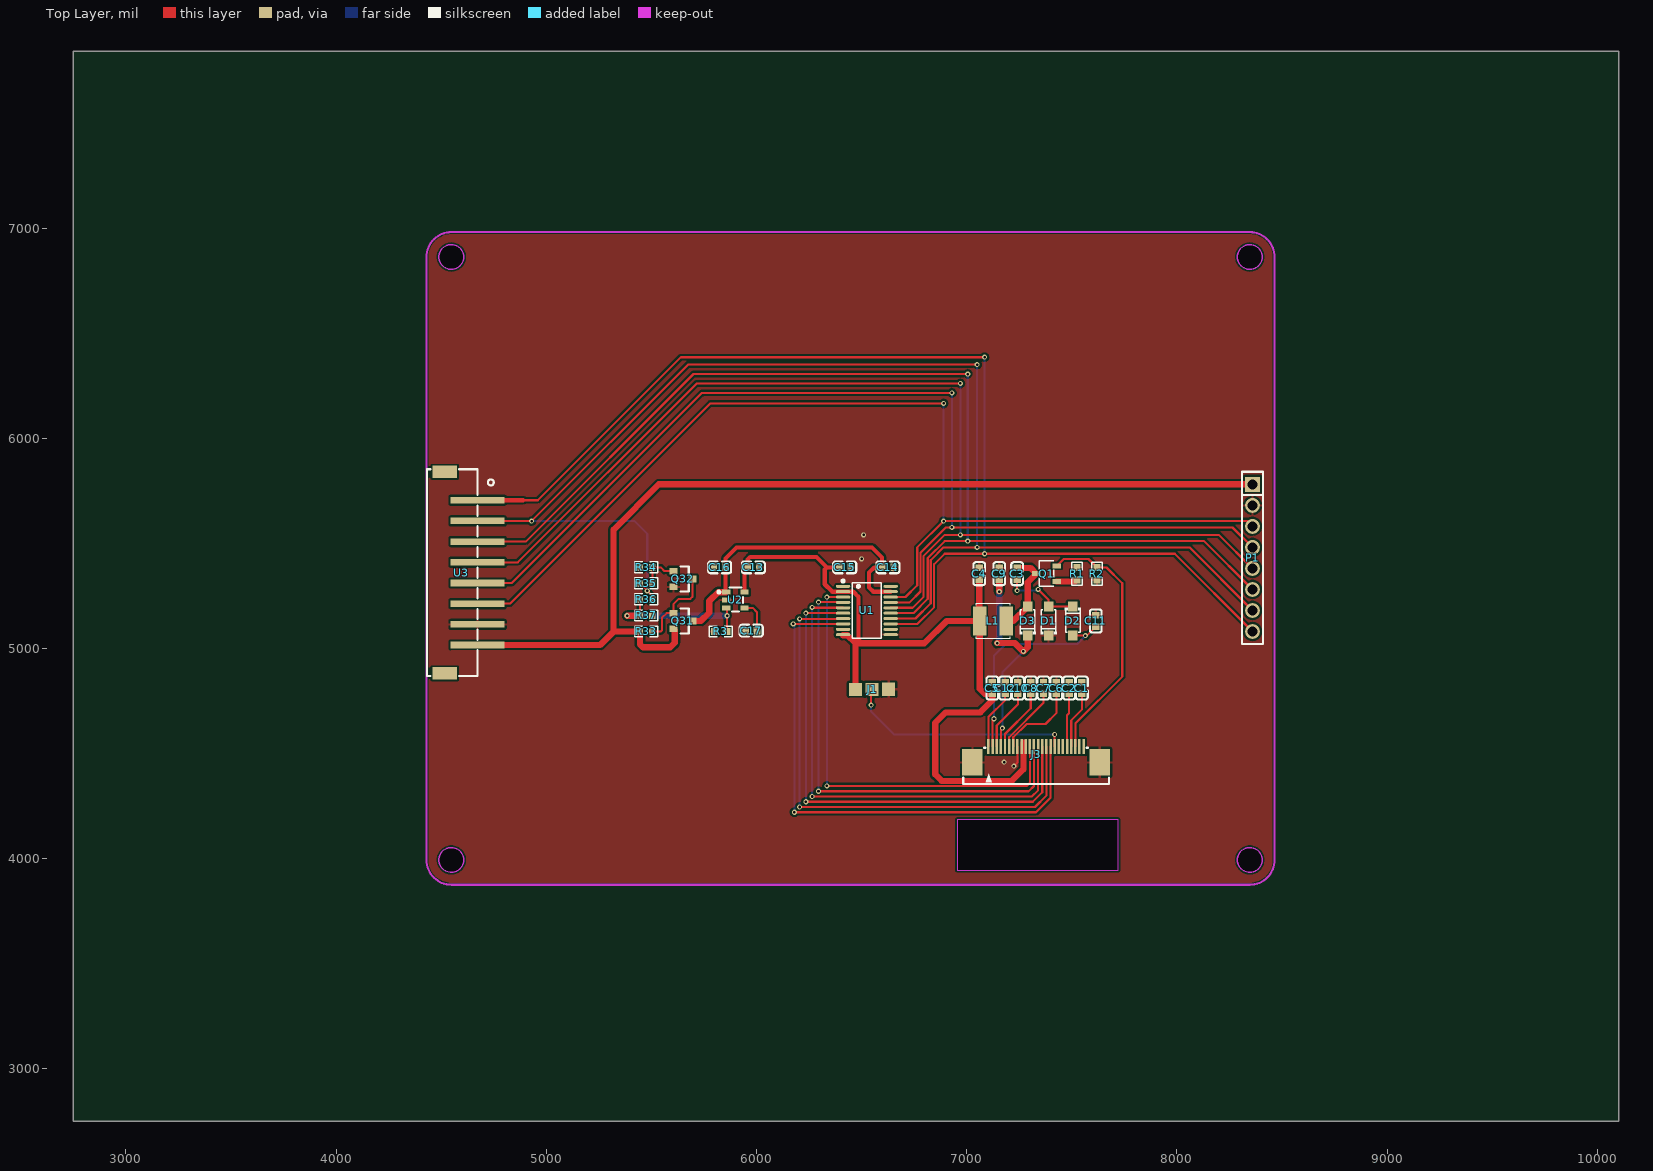
[diagram p0: Top Layer view]
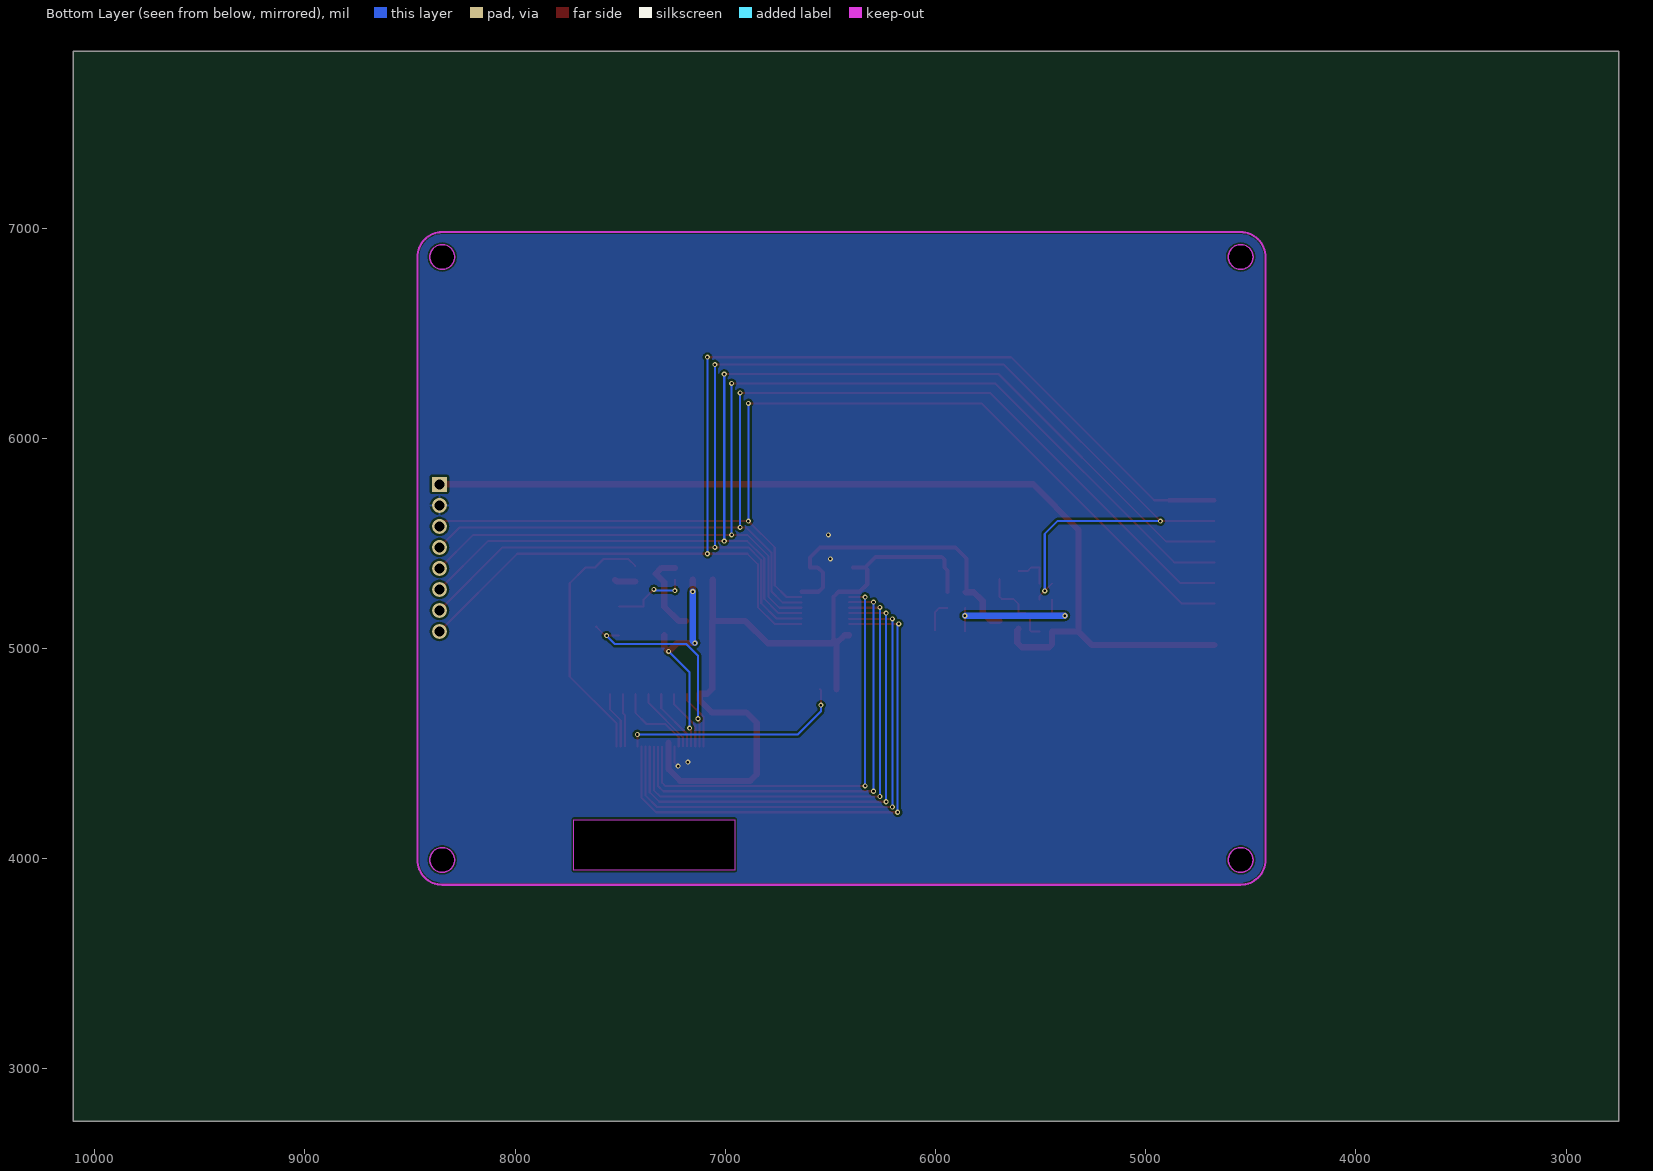
[diagram p1: Bottom Layer view, seen from below]
# Altium PCB MISC61435.pcbdoc
Units mil, origin at the board's own origin, x right, y up, seen from the top; angles counter-clockwise.
Board outline 7351.71 x 5090.35 mil, 2 copper layers (Top Layer, Bottom Layer), stack 62.206 mil thick; 38 components, 35 nets, 139 pads, 42 vias.

## Layer stack, top to bottom
Top Solder Mask Layer: solder mask 0.394, Dk 3.3
Top Layer: signal copper 1.379
Dielectric1: surface 59.449, FR4, Dk 4.5
Bottom Layer: signal copper 1.378
Bottom Solder Mask Layer: solder mask 0.394, Dk 3.3

## Board outline
10101.71,2750 2750,2750 2750,7840.35 10101.71,7840.35
cut-out: 4607.17,3993.46 cw(c4548.11,3993.46) 4489.06,3993.46 cw(c4548.11,3993.46)
cut-out: 8405.94,3993.46 cw(c8346.89,3993.46) 8287.83,3993.46 cw(c8346.89,3993.46)
cut-out: 8405.94,6862.24 cw(c8346.89,6862.24) 8287.83,6862.24 cw(c8346.89,6862.24)
cut-out: 4607.17,6862.24 cw(c4548.11,6862.24) 4489.06,6862.24 cw(c4548.11,6862.24)
cut-out: 6955,4185.35 6955,3945.35 7720,3945.35 7720,4185.35

## Design rules (kind name [scope] priority, off if disabled: settings)
BoardOutlineClearance copperThickness2oz_1 [All] p2 off: genericclearance=7.99 ignorepadtopadclearanceinfootprint=FALSE except(0: Arc-SplitContinuation Track-SplitContinuation SMDPad-SplitContinuation THPad-SplitContinuation Via-SplitContinuation Fill-SplitContinuation Region-SplitContinuation Poly-SplitContinuation Text-SplitContinuation Hole-SplitContinuation; 5.98: Arc-CutoutEdge SMDPad-CutoutEdge THPad-CutoutEdge Via-CutoutEdge Fill-CutoutEdge Region-CutoutEdge Text-CutoutEdge; 6.93: Hole-OutlineEdge Hole-CutoutEdge; 10: Poly-OutlineEdge Poly-CutoutEdge; 11.81: Arc-OutlineEdge Track-OutlineEdge SMDPad-OutlineEdge THPad-OutlineEdge Via-OutlineEdge Fill-OutlineEdge Region-OutlineEdge Text-OutlineEdge Track-CutoutEdge)
BoardOutlineClearance copperThickness1oz_1 [All] p4: genericclearance=4.02 ignorepadtopadclearanceinfootprint=FALSE except(0: Arc-SplitContinuation Track-SplitContinuation SMDPad-SplitContinuation THPad-SplitContinuation Via-SplitContinuation Fill-SplitContinuation Region-SplitContinuation Poly-SplitContinuation Text-SplitContinuation Hole-SplitContinuation; 6: SMDPad-CutoutEdge THPad-CutoutEdge Via-CutoutEdge Fill-CutoutEdge Region-CutoutEdge Text-CutoutEdge; 6.93: Hole-OutlineEdge Hole-CutoutEdge; 10: Poly-OutlineEdge Poly-CutoutEdge; 11.8: Arc-OutlineEdge Track-OutlineEdge SMDPad-OutlineEdge THPad-OutlineEdge Via-OutlineEdge Fill-OutlineEdge Region-OutlineEdge Text-OutlineEdge; 11.81: Arc-CutoutEdge Track-CutoutEdge)
Clearance copperThickness2oz [All] p1 off: gap=7.99 ignorepadtopadclearanceinfootprint=FALSE except(5.98: SMDPad-Track SMDPad-SMDPad THPad-Track SMDPad-THPad THPad-THPad Track-Via SMDPad-Via THPad-Via Via-Via Fill-Track Region-Track Fill-SMDPad Region-SMDPad Fill-THPad Region-THPad Fill-Via Region-Via Fill-Fill Fill-Region Region-Region Arc-Track Arc-SMDPad Arc-THPad Arc-Via Fill-Arc Region-Arc Arc-Arc Text-Track SMDPad-Text Text-THPad Text-Via Fill-Text Region-Text Arc-Text Text-Text; 6.93: Hole-Track Hole-SMDPad Hole-THPad Hole-Via Fill-Hole Region-Hole Hole-Arc Hole-Text; 10: Poly-Track Poly-SMDPad Poly-THPad Poly-Via Poly-Fill Poly-Region Poly-Poly Poly-Arc Poly-Text Poly-Hole)
Clearance copperThickness1oz [All] p3: gap=4.02 ignorepadtopadclearanceinfootprint=FALSE except(5.98: SMDPad-Track SMDPad-SMDPad THPad-Track SMDPad-THPad THPad-THPad Track-Via SMDPad-Via THPad-Via Via-Via Fill-Track Region-Track Fill-SMDPad Region-SMDPad Fill-THPad Region-THPad Fill-Via Region-Via Fill-Fill Fill-Region Region-Region; 6: Arc-Track Arc-SMDPad Arc-THPad Arc-Via Fill-Arc Region-Arc Arc-Arc Text-Track SMDPad-Text Text-THPad Text-Via Fill-Text Region-Text Arc-Text Text-Text; 6.93: Hole-Track Hole-SMDPad Hole-THPad Hole-Via Fill-Hole Region-Hole Hole-Arc Hole-Text; 10: Poly-Track Poly-SMDPad Poly-THPad Poly-Via Poly-Fill Poly-Region Poly-Poly Poly-Arc Poly-Text Poly-Hole)
DiffPairsRouting differentialPair [All] p1: maxlimit=6 minlimit=6 mostfreqgap=6 toplayer_minwidth=5 toplayer_prefwidth=10 toplayer_maxwidth=100 toplayer_mingap=6 toplayer_prefgap=6 toplayer_maxgap=6 bottomlayer_minwidth=5 bottomlayer_prefwidth=10 bottomlayer_maxwidth=100 bottomlayer_mingap=6 bottomlayer_prefgap=6 bottomlayer_maxgap=6 maxuncoupledlength=10
HoleToHoleClearance otherClearance [All] p1: gap=11.81 allowstackedmicrovias=TRUE
Length netLength [All] p1: minlimit=0 maxlimit=0
MatchedLengths netLengthTolerance [All] p1: tolerance=1000
PasteMaskExpansion pasteMaskExpansion [All] p1: expansion=0
PlaneConnect innerPlane [All] p1: planeconnectstyle=Relief reliefexpansion=20 reliefentries=4 reliefconductorwidth=10 reliefairgap=10
PolygonConnect copperRegion [(InNet('GND'))] p1: connectstyle=Relief reliefconductorwidth=10 reliefentries=4 polygonreliefangle="90 Angle" airgapwidth=10 via.connectstyle=Relief via.reliefconductorwidth=10 via.reliefentries=4 via.polygonreliefangle="90 Angle" via.airgapwidth=10
RoutingVias viaSize [All] p1: holewidth=12.01 width=24.02 viastyle="Through Hole" minholewidth=11.81 minwidth=19.68 maxholewidth=248.03 maxwidth=393.7
SolderMaskExpansion solderMaskExpansion [IsVia] p1: expansion=-1000 istentingtop=TRUE
SolderMaskExpansion solderMaskExpansion [All] p2: expansion=2 istentingtop=FALSE
Width copperThickness2oz_2 [All] p1 off: maxlimit=100 minlimit=8 preferedwidth=10
Width copperThickness1oz_2 [All] p2: maxlimit=100 minlimit=5 preferedwidth=10

## Components (designator, comment, footprint, x,y, rotation, side; value= is the part's Value field where it differs from the comment)
C1 "1uF" C0603 7548.08,4811.22 r270 top
C2 "1uF" C0603 7487.24,4811.22 r270 top
C3 "4.7uF" C0603 7240,5355.34 r90 top
C4 "4.7uF" C0603 7060,5355.34 r270 top
C5 "1uF" C0603 7122.19,4811.22 r270 top
C6 "1uF" C0603 7426.4,4811.22 r270 top
C7 "1uF" C0603 7365.56,4811.22 r270 top
C8 "1uF" C0603 7304.71,4811.22 r270 top
C9 "1uF" C0603 7155,5355.35 r270 top
C10 "1uF" C0603 7243.87,4811.22 r270 top
C11 "1uF" C0603 7613.97,5130.33 r270 top
C12 "1uF" C0603 7183.03,4811.22 r270 top
C13 "100nF" C0603 5985,5385.35 r180 top
C14 "100nF" C0603 6625,5385.35 r0 top
C15 "100nF" C0603 6420,5385.35 r0 top
C16 "1uF" C0603 5824.92,5385.35 r0 top
C17 "22nF" C0603 5975,5084.29 r0 top
D1 "MBR0530" SOD-123FL_L2.7-W1.8-LS3.7-RD 7390,5130.33 r90 top
D2 "MBR0530" SOD-123FL_L2.7-W1.8-LS3.7-RD 7505,5130.33 r270 top
D3 "MBR0530" SOD-123FL_L2.7-W1.8-LS3.7-RD 7290,5130.33 r90 top
J1 "" HDR-TH_3P-P2.54-V-F 6550,4805.35 r0 top
J3 "FPC0.5-24P/top-entry pull-out" FPC-SMD_24P-P0.50_SHOU-HAN_CTSJ-H2.0 7330,4495.35 r0 top
L1 "GCNR4018" IND-SMD_L4.0-W4.0 7125,5130.35 r0 top
P1 "" HDR-TH_8P-P2.54-V-F-1 8360,5430.35 r270 top
Q1 "BSS138LT1G" SOT-23-3_L2.9-W1.6-P1.90-LS2.8-BR 7380,5355.35 r0 top
Q31 "SI2301CDS-T1-E3" SOT-23_L2.9-W1.3-P1.90-LS2.4-BR 5650,5130.35 r180 top
Q32 "" S8050_SOT-23 5650,5330.35 r180 top
R1 "10K" R0603 7525,5355.35 r90 top
R2 "10K" R0603 7620,5355.35 r270 top
R3 "100K" R0603 5830,5080.35 r0 top
R33 "100K" R0603 5475,5080.35 r180 top
R34 "47K" R0603 5475,5385.35 r0 top
R35 "1K" R0603 5475,5309.1 r0 top
R36 "1K" R0603 5475,5232.85 r0 top
R37 "47K" R0603 5475,5156.6 r0 top
U1 "TXB0108PWR" TSSOP-20_L6.5-W4.4-P0.65-LS6.4-BL 6525,5180.35 r270 top
U2 "RT9193-33GB-MS" SOT-23-5_L2.9-W1.6-P0.95-LS2.8-BR 5900,5230.35 r180 top
U3 "XH2.54-LS-8P" CONN-SMD_XH2.54-LS-8P 4595,5360.35 r270 top

## Footprints (in the part's own frame and the unit in brackets; to place one, negate y for a bottom-side part, rotate by r counter-clockwise, add the part's x,y. Pads: shape width x height; smd on the part's side, far side on the other; paste and mask are expansions set on the pad)
C0603 [mm]
  rect 0.8x0.9 smd: 1(-0.7,0) 2(0.7,0)
  silkscreen extent -1.39,-0.71 1.39,0.71
CONN-SMD_XH2.54-LS-8P [mm]
  rect 0.8x6.5 smd paste+0 mask+0.05: 1(-8.75,1.984) 2(-6.25,1.984) 3(-3.75,1.984) 4(-1.25,1.984) 5(1.25,1.984) 6(3.75,1.984) 7(6.25,1.984) 8(8.75,1.984)
  rect 1.5x3 smd paste+0 mask+0.05: 9(-12.17,-1.985) 10(12.17,-1.985)
  silkscreen extent -12.5,-4.12 12.5,3.94
FPC-SMD_24P-P0.50_SHOU-HAN_CTSJ-H2.0 [mm]
  rect 0.3x1.8 smd paste+0 mask+0.05: 1(-5.75,0.95) 2(-5.25,0.95) 3(-4.75,0.95) 4(-4.25,0.95) 5(-3.75,0.95) 6(-3.25,0.95) 7(-2.75,0.95) 8(-2.25,0.95) 9(-1.75,0.95) 10(-1.25,0.95) 11(-0.75,0.95) 12(-0.25,0.95) 13(0.25,0.95) 14(0.75,0.95) 15(1.25,0.95) 16(1.75,0.95) 17(2.25,0.95) 18(2.75,0.95) 19(3.25,0.95) 20(3.75,0.95) 21(4.25,0.95) 22(4.75,0.95) 23(5.25,0.95) 24(5.75,0.95)
  rect 2.5x3.2 smd paste+0 mask+0.05: 25(7.7,-0.95) 26(-7.7,-0.95)
  silkscreen extent -8.8,-3.59 8.8,0.81
HDR-TH_3P-P2.54-V-F [mil]
  rect 62x62 smd: 1(-78.5,-0.28) 2(0,0) 3(79.02,0.28)
HDR-TH_8P-P2.54-V-F-1 [mm]
  rect 1.8x1.8 hole 1.2: 1(-8.89,0)
  round 1.8 hole 1.2: 2(-6.35,0) 3(-3.81,0) 4(-1.27,0) 5(1.27,0) 6(3.81,0) 7(6.35,0) 8(8.89,0)
  silkscreen extent -10.41,-1.25 10.41,1.25
IND-SMD_L4.0-W4.0 [mm]
  rect 1.6x3.5 smd: 1(-1.6,0) 2(1.6,0)
  silkscreen extent -2.08,-2.1 2.08,2.1
R0603 [mil]
  rect 31.75x34.02 smd paste-3937.01 mask+2: 1(-29.66,0) 2(29.66,0)
  silkscreen extent -55,-26 55,26
S8050_SOT-23 [mm]
  rect 1x0.8 smd paste+0 mask+0.051: 1(1.15,-0.95) 2(1.15,0.95) 3(-1.15,0)
  silkscreen extent -0.7,-1.5 0.7,1.5
SOD-123FL_L2.7-W1.8-LS3.7-RD [mm]
  rect 1.2x1.15 smd: 1(-1.735,0) 2(1.735,0)
  silkscreen extent -1.6,-0.95 1.38,0.95
SOT-23-3_L2.9-W1.6-P1.90-LS2.8-BR [mm]
  rect 1.07x0.6 smd: 1(1.235,-0.95) 2(1.235,0.95) 3(-1.235,0)
  silkscreen extent -0.88,-1.54 0.88,1.54
SOT-23-5_L2.9-W1.6-P0.95-LS2.8-BR [mm]
  rect 1x0.6 smd paste+0 mask+0.05: 1(1.1,-0.95) 2(1.1,0) 3(1.1,0.95) 4(-1.1,0.95) 5(-1.1,-0.95)
  silkscreen extent -0.89,-1.52 2.16,1.4
SOT-23_L2.9-W1.3-P1.90-LS2.4-BR [mm]
  rect 1x0.8 smd: 1(1.15,-0.95) 2(1.15,0.95) 3(-1.15,0)
  silkscreen extent -0.7,-1.5 0.7,1.5
TSSOP-20_L6.5-W4.4-P0.65-LS6.4-BL [mil]
  oval 14.33x68.58 smd: 1(-115.16,-113.03) 2(-89.57,-113.03) 3(-63.98,-113.03) 4(-38.39,-113.03) 5(-12.79,-113.03) 6(12.8,-113.03) 7(38.39,-113.03) 8(63.98,-113.03) 9(89.57,-113.03) 10(115.16,-113.03) 11(115.16,113.03) 12(89.57,113.03) 13(63.98,113.03) 14(38.39,113.03) 15(12.8,113.03) 16(-12.79,113.03) 17(-38.39,113.03) 18(-63.98,113.03) 19(-89.57,113.03) 20(-115.16,113.03)
  silkscreen extent -146,-119 131,70

## Via types
v1: diameter 24.02, hole 12, Top Layer to Bottom Layer, 42 vias

## Nets (pads, with @x,y where several pads share a name; then routed paths per layer and width w, separated by ;. In a path a pad name is that pad's centre, name@x,y a point inside that pad or via, vN(x,y) a via of type N, cw(c..) or ccw(c..) an arc to the next point about the centre after c; other vN are vias at no path point)
3V3: C4.2 C5.2 C13.2 C15.1 J1.1 J3.9 J3.10 L1.1 U1.2 U1.10 U2.5 | length 3811.3
  Top Layer w20: U2.5 5943.31,5371.22 C13.2 5957.44,5422.79 5970,5435.35 6285,5435.35 6335,5385.35 ; C15.1 6335,5385.35 ; 6485,5037.35 6485,5245.35 6460.43,5269.92 U1.2 6360.43,5269.92 6325,5305.35 6325,5375.35 6335,5385.35
  Top Layer w30: U1.10@6411.97,5062.63 6432.72,5062.63 6471.5,5023.85 ; J1.1 6471.5,5023.85 ; 6485,5037.35 6471.5,5023.85 ; C4.2 7060,5132.36 L1.1 ; 7270,4550.35 7270,4425.35 7214.02,4369.36 6880.98,4369.36 6850,4400.35 6850,4645.35 6900,4695.35 7065,4695.35 7122.19,4752.53 C5.2 7086.68,4783.66 7062.01,4808.34 L1.1 ; 6471.5,5023.85 6798.5,5023.85 6905,5130.35 L1.1
$1N5: C3.2 D3.2 L1.2 Q1.3 | length 406.9
  Top Layer w30: L1.2 7221.71,5130.35 D3.2 7290,5313.97 Q1.3 7303.82,5382.9 C3.2
$1N8: C3.1 D1.2 D2.1 | length 371.9
  Top Layer w10: v1(7240,5275.35) C3.1 ; v1(7340,5280.35) 7390,5230.35 D1.2 D2.1
  Bottom Layer w10: v1(7240,5275.35) 7335,5275.35 v1(7340,5280.35)
$1N13: Q1.1 R1.1 | length 99.6
  Top Layer w30: Q1.1 7517.26,5317.95 R1.1
$1N30: C1.2 J3.21 | length 271.9
  Top Layer w10: J3.21 7497.32,4657.67 7548.08,4708.43 C1.2
$1N31: C2.2 J3.20 | length 254.9
  Top Layer w10: J3.20 7477.64,4682.99 7487.24,4692.59 C2.2
$1N34: C6.2 J3.7 | length 388.4
  Top Layer w10: J3.7 7221.73,4577.08 7285,4640.35 7375,4640.35 7426.4,4691.74 C6.2
$1N35: C7.2 J3.6 | length 318.6
  Top Layer w10: J3.6 7202.05,4577.4 7365.56,4740.9 C7.2
$1N36: C8.2 J3.5 | length 301.6
  Top Layer w10: J3.5 7182.36,4592.71 7304.71,4715.06 C8.2
$1N37: C10.2 J3.3 | length 292.7
  Top Layer w10: J3.3 7142.99,4633.34 7243.87,4734.22 C10.2
$1N38: C12.2 J3.1 | length 283.8
  Top Layer w10: J3.1 7103.62,4673.97 7183.03,4753.38 C12.2
$1N65: Q31.1 Q32.3 R33.1 | length 403.7
  Top Layer w10: R33.1 5545,5080.35 5550,5085.35 5550,5145.35 5572.4,5167.75 Q31.1 5604.73,5210.07 5630,5235.35 5685,5235.35 5695.28,5245.62 Q32.3
$1N66: Q32.1 R34.2 R35.2 | length 183.6
  Top Layer w10: R35.2 R34.2 5545,5385.35 5562.6,5367.75 Q32.1
$1N76: C17.2 U2.4 | length 156.1
  Top Layer w10: U2.4 5982.4,5192.94 6002.56,5172.79 C17.2
BS: J1.2 J3.17 | length 1083.8
  Top Layer w10: v1(6545,4730.35) 6545,4800.35 J1.2 ; J3.17 v1(7418.58,4590.35)
  Bottom Layer w10: v1(6545,4730.35) 6545,4700.35 6655,4590.35 v1(7418.58,4590.35)
BUSY: P1.8 U1.13 U3.1 | length 5762.4
  Top Layer w10: 4889.49,5704.84 4959.49,5704.84 5640,6385.35 v1(7085,6385.35) ; U1.13 6766.02,5116.37 6845,5195.35 6845,5400.35 6895,5450.35 v1(7085,5450.35) 7990,5450.35 P1.8
  Top Layer w20: U3.1 4889.49,5704.84
  Bottom Layer w10: v1(7085,5450.35) v1(7085,6385.35)
BUSY': J3.16 U1.8 | length 2626
  Top Layer w10: v1(6175,5116.37) U1.8 ; v1(6180,4220.35) 7330,4220.35 7398.9,4289.25 J3.16
  Bottom Layer w10: v1(6175,5116.37) 6180,5111.37 v1(6180,4220.35)
CLK: P1.4 U1.17 U3.5 | length 5288.8
  Top Layer w10: U3.5 4835.79,5311.14 5740,6215.35 v1(6930,6215.35) ; U1.17 6728.39,5218.74 6780,5270.35 6780,5455.35 6900,5575.35 v1(6930,5575.35) 8265,5575.35 P1.4
  Bottom Layer w10: v1(6930,5575.35) v1(6930,6215.35)
CLK': J3.12 U1.4 | length 2240.5
  Top Layer w10: v1(6295,4320.35) 7295,4320.35 7320.16,4345.51 J3.12 ; v1(6295,5220.35) 6410.36,5220.35 U1.4
  Bottom Layer w10: v1(6295,4320.35) v1(6295,5220.35)
CS: P1.5 U1.16 U3.4 | length 5415.6
  Top Layer w10: U3.4 4864.21,5409.56 5715,6260.35 v1(6970,6260.35) ; U1.16 6742.79,5193.14 6795,5245.35 6795,5440.35 6895,5540.35 v1(6970,5540.35) 8200,5540.35 P1.5
  Bottom Layer w10: v1(6970,5540.35) v1(6970,6260.35)
CS': J3.13 U1.5 | length 2342.6
  Top Layer w10: v1(6265,4295.35) 7310,4295.35 7339.84,4325.19 J3.13 ; v1(6265,5195.35) 6267.21,5193.14 U1.5
  Bottom Layer w10: v1(6265,4295.35) v1(6265,5195.35)
D/C: P1.6 U1.15 U3.3 | length 5530.6
  Top Layer w10: U3.3 4902.64,5507.99 5700,6305.35 v1(7005,6305.35) ; U1.15 6747.2,5167.55 6815,5235.35 6815,5430.35 6895,5510.35 v1(7005,5510.35) 8130,5510.35 P1.6
  Bottom Layer w10: v1(7005,5510.35) v1(7005,6305.35)
D/C': J3.14 U1.6 | length 2435
  Top Layer w10: v1(6235,4270.35) 7315,4270.35 7359.53,4314.88 J3.14 ; v1(6235,5167.55) U1.6
  Bottom Layer w10: v1(6235,4270.35) v1(6235,5167.55)
DIN: P1.3 U1.18 U3.6 | length 5158.8
  Top Layer w10: U3.6 4827.36,5212.71 5780,6165.35 v1(6890,6165.35) ; U1.18 6708.98,5244.33 6765,5300.35 6765,5480.35 v1(6890,5605.35) 8335,5605.35 P1.3
  Bottom Layer w10: v1(6890,5605.35) v1(6890,6165.35)
DIN': J3.11 U1.3 | length 2119.8
  Top Layer w10: v1(6335,4345.35) 7285,4345.35 7300.47,4360.82 J3.11 ; v1(6335,5244.33) U1.3
  Bottom Layer w10: v1(6335,4345.35) v1(6335,5244.33)
GDR: J3.23
GND: C4.1 C5.1 C6.1 C7.1 C8.1 C9.1 C10.1 C11.1 C12.1 C13.1 C14.2 C15.2 C16.1 C17.1 D1.1 J1.3 J3.8 J3.25 J3.26 P1.2 Q32.2 R1.2 R2.2 R3.1 R34.1 R37.2 U1.11 U2.2 U3.7 | length 99.2
  Top Layer w10: v1(7225,4440.35) 7241.42,4456.77 J3.8
  other v1: 7178.09,4458.63 6500,5425.35 6510,5540.35
PREVGH: C9.2 D3.1 J3.4 | length 1030.2
  Top Layer w10: J3.4 7162.68,4613.03 v1(7170,4620.35)
  Top Layer w30: v1(7145,5025.35) 7230,5025.35 v1(7270,4985.35) 7290,5005.35 D3.1 ; v1(7155,5270.35) C9.2
  Bottom Layer w10: v1(7170,4620.35) 7170,4885.35 v1(7270,4985.35)
  Bottom Layer w30: v1(7145,5025.35) 7155,5035.35 v1(7155,5270.35)
PREVGL: C11.2 D2.2 J3.2 | length 1035.6
  Top Layer w10: J3.2 7123.31,4658.66 v1(7130,4665.35) ; D2.2 7573.23,5062.03 C11.2
  Bottom Layer w10: v1(7130,4665.35) 7130,4965.35 7185,5020.35 7525,5020.35 v1(7565,5060.35)
RESE: J3.22 Q1.2 R2.1 | length 1242.5
  Top Layer w10: Q1.2 7461.23,5425.35 7579.66,5425.35 R2.1 7665.34,5385.01 7740,5310.35 7740,4865.35 7517.01,4642.36 J3.22
RST: P1.7 R35.1 R36.2 U1.14 U3.2 | length 6608.6
  Top Layer w10: U3.2 4931.06,5606.41 5675,6350.35 v1(7050,6350.35) ; R35.1 v1(5480.36,5274.08) 5504.66,5249.78 R36.2 ; U1.14 6756.61,5141.96 6829.02,5214.36 6829.02,5419.36 6890,5480.35 v1(7050,5480.35) 8060,5480.35 P1.7
  Bottom Layer w10: v1(4930,5605.35) 5420,5605.35 5480.36,5544.99 v1(5480.36,5274.08) ; v1(7050,5480.35) v1(7050,6350.35)
RST': J3.15 U1.7 | length 2532.5
  Top Layer w10: v1(6205,4245.35) 7325,4245.35 7379.21,4299.56 J3.15 ; v1(6205,5140.35) 6410.36,5140.35 U1.7
  Bottom Layer w10: v1(6205,4245.35) v1(6205,5140.35)
VCC: C14.1 C16.2 Q31.3 U1.19 U2.1 | length 1500.6
  Top Layer w20: U2.1 5852.48,5271.95 C16.2 5852.48,5427.83 5905,5480.35 6550,5480.35 6597.44,5432.91 C14.1 6560,5385.35 6535,5360.35 6535,5290.35 6555.43,5269.92 U1.19
  Top Layer w30: Q31.3 5735,5130.35 5775,5170.35 5775,5225.35 5817.4,5267.74 U2.1
VCC_EN: R3.2 R36.1 R37.1 U2.3 | length 725.9
  Top Layer w10: R37.1 R36.1 ; U2.3 5859.66,5189.98 R3.2
  Top Layer w30: v1(5385,5155.35) 5444.09,5155.35 R37.1
  Bottom Layer w30: v1(5385,5155.35) v1(5860,5155.35)
VCC_INT: P1.1 Q31.2 R33.2 U3.8 | length 4723.1
  Top Layer w30: U3.8 5255.51,5015.86 5320,5080.35 ; Q31.2 5611.21,5086.46 5611.21,5026.56 5590,5005.35 5460,5005.35 5445.34,5020.01 R33.2 5320,5080.35 ; P1.1 5535,5780.35 5320,5565.35 5320,5080.35
pads on no net: C1.1 C2.1 J3.18 J3.19 J3.24 U1.1 U1.9 U1.12 U1.20 U3.9 U3.10

## Polygon pours and split planes (outlines as drawn)
GND on Top Layer (solid, remove dead copper, pour order 0): 3970,7590.35 3970,3335.35 8975,3335.35 8975,7590.35
GND on Bottom Layer (solid, remove dead copper, pour order 2): 4285,7365.35 4285,3315.35 8760,3315.35 8760,7365.35

## Keep-outs
Board Outline Layer:
  region: 4607.17,3993.46 cw(c4548.11,3993.46) 4489.06,3993.46 cw(c4548.11,3993.46)
  circle w0.1: c4548.11,3993.46 r59.06
  region: 4607.17,3993.46 4606.77,3986.6 4605.57,3979.84 4603.6,3973.26 4600.88,3966.95 4597.45,3961 4593.35,3955.5 4588.64,3950.5 4583.38,3946.09 4577.64,3942.31 4571.5,3939.23 4565.05,3936.88 4558.36,3935.3 4551.54,3934.5 4544.68,3934.5 4537.86,3935.3 4531.17,3936.88 4524.72,3939.23 4518.58,3942.31 4512.84,3946.09 4507.58,3950.5 4502.87,3955.5 4498.77,3961 4495.34,3966.95 4492.62,3973.26 4490.65,3979.84 4489.45,3986.6 4489.06,3993.46 4489.45,4000.31 4490.65,4007.07 4492.62,4013.65 4495.34,4019.96 4498.77,4025.91 4502.87,4031.42 4507.58,4036.41 4512.84,4040.83 4518.58,4044.6 4524.72,4047.68 4531.17,4050.03 4537.86,4051.61 4544.68,4052.41 4551.54,4052.41 4558.36,4051.61 4565.05,4050.03 4571.5,4047.68 4577.64,4044.6 4583.38,4040.83 4588.64,4036.41 4593.35,4031.42 4597.45,4025.91 4600.88,4019.96 4603.6,4013.65 4605.57,4007.07 4606.77,4000.31
  region: 8405.94,3993.46 cw(c8346.89,3993.46) 8287.83,3993.46 cw(c8346.89,3993.46)
  circle w0.1: c8346.89,3993.46 r59.06
  region: 8405.94,3993.46 8405.55,3986.6 8404.35,3979.84 8402.38,3973.26 8399.66,3966.95 8396.23,3961 8392.13,3955.5 8387.42,3950.5 8382.16,3946.09 8376.42,3942.31 8370.28,3939.23 8363.83,3936.88 8357.14,3935.3 8350.32,3934.5 8343.46,3934.5 8336.64,3935.3 8329.95,3936.88 8323.5,3939.23 8317.36,3942.31 8311.62,3946.09 8306.36,3950.5 8301.65,3955.5 8297.55,3961 8294.12,3966.95 8291.4,3973.26 8289.43,3979.84 8288.23,3986.6 8287.83,3993.46 8288.23,4000.31 8289.43,4007.07 8291.4,4013.65 8294.12,4019.96 8297.55,4025.91 8301.65,4031.42 8306.36,4036.41 8311.62,4040.83 8317.36,4044.6 8323.5,4047.68 8329.95,4050.03 8336.64,4051.61 8343.46,4052.41 8350.32,4052.41 8357.14,4051.61 8363.83,4050.03 8370.28,4047.68 8376.42,4044.6 8382.16,4040.83 8387.42,4036.41 8392.13,4031.42 8396.23,4025.91 8399.66,4019.96 8402.38,4013.65 8404.35,4007.07 8405.55,4000.31
  region: 8405.94,6862.24 cw(c8346.89,6862.24) 8287.83,6862.24 cw(c8346.89,6862.24)
  circle w0.1: c8346.89,6862.24 r59.06
  region: 8405.94,6862.24 8405.55,6855.38 8404.35,6848.62 8402.38,6842.04 8399.66,6835.73 8396.23,6829.78 8392.13,6824.28 8387.42,6819.28 8382.16,6814.87 8376.42,6811.09 8370.28,6808.01 8363.83,6805.66 8357.14,6804.08 8350.32,6803.28 8343.46,6803.28 8336.64,6804.08 8329.95,6805.66 8323.5,6808.01 8317.36,6811.09 8311.62,6814.87 8306.36,6819.28 8301.65,6824.28 8297.55,6829.78 8294.12,6835.73 8291.4,6842.04 8289.43,6848.62 8288.23,6855.38 8287.83,6862.24 8288.23,6869.09 8289.43,6875.85 8291.4,6882.43 8294.12,6888.74 8297.55,6894.69 8301.65,6900.2 8306.36,6905.19 8311.62,6909.61 8317.36,6913.38 8323.5,6916.46 8329.95,6918.81 8336.64,6920.39 8343.46,6921.19 8350.32,6921.19 8357.14,6920.39 8363.83,6918.81 8370.28,6916.46 8376.42,6913.38 8382.16,6909.61 8387.42,6905.19 8392.13,6900.2 8396.23,6894.69 8399.66,6888.74 8402.38,6882.43 8404.35,6875.85 8405.55,6869.09
  region: 4607.17,6862.24 cw(c4548.11,6862.24) 4489.06,6862.24 cw(c4548.11,6862.24)
  circle w0.1: c4548.11,6862.24 r59.06
  region: 4607.17,6862.24 4606.77,6855.38 4605.57,6848.62 4603.6,6842.04 4600.88,6835.73 4597.45,6829.78 4593.35,6824.28 4588.64,6819.28 4583.38,6814.87 4577.64,6811.09 4571.5,6808.01 4565.05,6805.66 4558.36,6804.08 4551.54,6803.28 4544.68,6803.28 4537.86,6804.08 4531.17,6805.66 4524.72,6808.01 4518.58,6811.09 4512.84,6814.87 4507.58,6819.28 4502.87,6824.28 4498.77,6829.78 4495.34,6835.73 4492.62,6842.04 4490.65,6848.62 4489.45,6855.38 4489.06,6862.24 4489.45,6869.09 4490.65,6875.85 4492.62,6882.43 4495.34,6888.74 4498.77,6894.69 4502.87,6900.2 4507.58,6905.19 4512.84,6909.61 4518.58,6913.38 4524.72,6916.46 4531.17,6918.81 4537.86,6920.39 4544.68,6921.19 4551.54,6921.19 4558.36,6920.39 4565.05,6918.81 4571.5,6916.46 4577.64,6913.38 4583.38,6909.61 4588.64,6905.19 4593.35,6900.2 4597.45,6894.69 4600.88,6888.74 4603.6,6882.43 4605.57,6875.85 4606.77,6869.09
  region: 6955,4185.35 6955,3945.35 7720,3945.35 7720,4185.35
  region: 6955,4185.35 6955,3945.35 7720,3945.35 7720,4185.35
  lines w0.1: 6955,3945.35 6955,4185.35 7720,4185.35 7720,3945.35 6955,3945.35
  lines w10: 4430,3993.46 4430,6862.24 cw(c4548.11,6862.24) 4548.11,6980.35 8346.89,6980.35 cw(c8346.89,6862.24) 8465,6862.24 8465,3993.46 cw(c8346.89,3993.46) 8346.89,3875.35 4548.11,3875.35 cw(c4548.11,3993.46) 4430,3993.46

## Silkscreen, mask and mechanical layers (free items; w line width, h text height)
Mechanical Layer:
  circle w0.1: c4548.11,3993.46 r59.06
  circle w0.1: c8346.89,3993.46 r59.06
  circle w0.1: c8346.89,6862.24 r59.06
  circle w0.1: c4548.11,6862.24 r59.06
  lines w0.1: 6955,3945.35 6955,4185.35 7720,4185.35 7720,3945.35 6955,3945.35